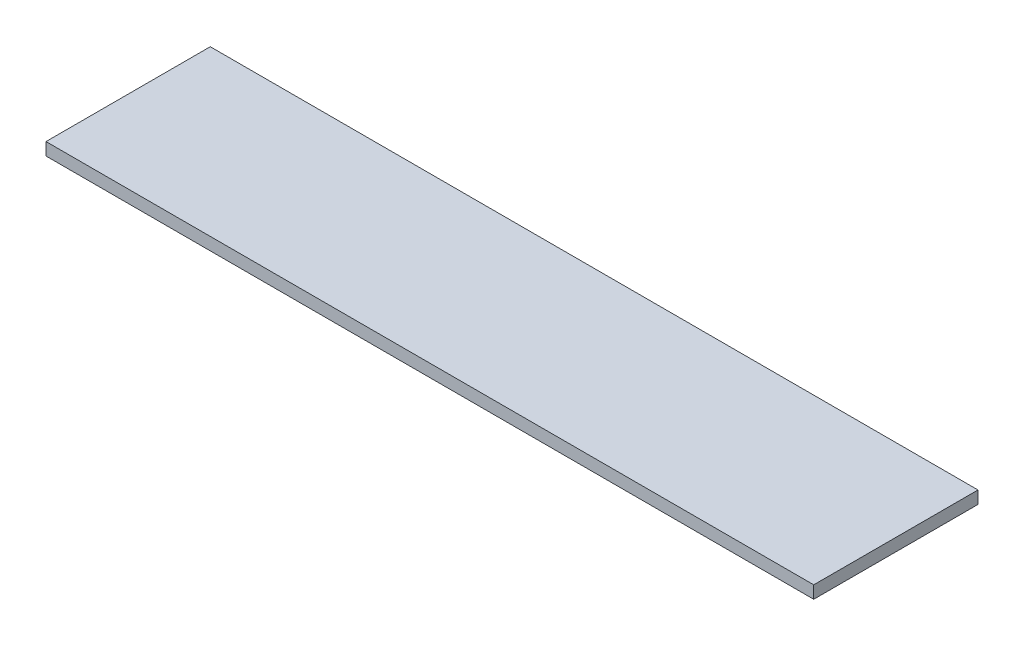
SolidWorks part; units mm, degrees
ref_plane "前视" through (0, 0, 0) normal (0, 0, 1) x (1, 0, 0)
ref_plane "上视" through (0, 0, 0) normal (0, 1, 0) x (1, 0, 0)
ref_plane "右视" through (0, 0, 0) normal (1, 0, 0) x (0, 0, -1)
sketch "草图1" plane through (0, 0, 0) normal (0, 1, 0) x (1, 0, 0)
  line L0 (0, 0) -> (0, 54.3289) construction
  line L1 (0, 0) -> (58.3533, 0) construction
  line L3 (-673, 144) -> (673, 144)
  line L4 (-673, 144) -> (-673, -144)
  line L5 (-673, -144) -> (673, -144)
  line L6 (673, 144) -> (673, -144)
  dimension "D1" = 1346
  dimension "D2" = 288
  dimension "D3" = 673
  dimension "D4" = 144
extrude "凸台-拉伸1" add sketch "草图1" against normal blind 20
shell "抽壳1" thickness 2
sketch "草图2" plane through (0, -20, 0) normal (0, -1, 0) x (1, 0, 0)
  line L1 (-673, 144) -> (673, 144)
  line L2 (-673, 144) -> (-673, -144)
  line L3 (-673, -144) -> (673, -144)
  line L4 (673, 144) -> (673, -144)
extrude "凸台-拉伸2" add sketch "草图2" along normal blind 2
